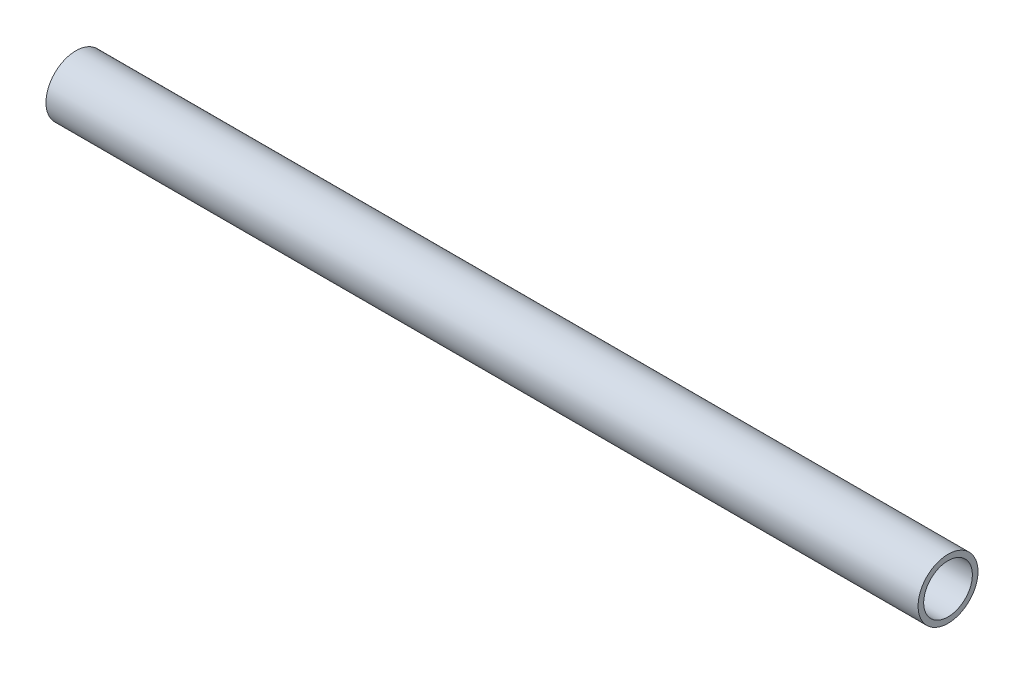
SolidWorks part; units mm, degrees
ref_plane "Front Plane" through (0, 0, 0) normal (0, 0, 1) x (1, 0, 0)
ref_plane "Top Plane" through (0, 0, 0) normal (0, 1, 0) x (1, 0, 0)
ref_plane "Right Plane" through (0, 0, 0) normal (1, 0, 0) x (0, 0, -1)
other "Configuration Table"
sketch "草图1" plane through (0, 0, 0) normal (0, 1, 0) x (1, 0, 0)
  line L0 (-155, 0) -> (155, 0)
  point P4 (0, 0)
  dimension "D1" = 310
other "Gb／t6728-2002 round tube 021.3 X 2 (1)"
ref_plane "Plane1" through (-155, 0, 0) normal (1, 0, 0) x (0, 0, -1)
sketch "Sketch1" plane through (-155, 0, 0) normal (1, 0, 0) x (0, 0, -1)
  circle A0 centre (0, 0) radius 8.65
  circle A1 centre (0, 0) radius 10.65
  point P3 (0, 0)
  dimension "In_dia" = 17.3
  dimension "Out_dia" = 21.3
